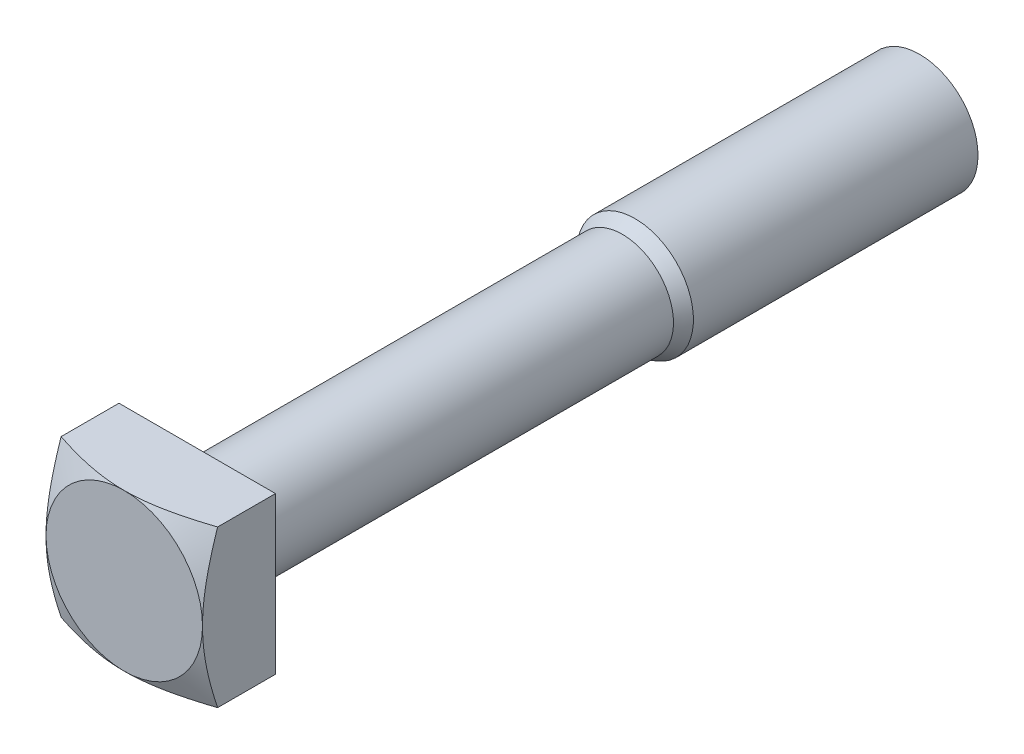
SolidWorks part; units mm, degrees
extrude "Base-Extrude" add sketch "Sketch1" along normal blind 15
sketch "Sketch1" plane through (0, 0, 0) normal (0, 0, 1) x (1, 0, 0)
  line L0 (-16.0867, 16.0867) -> (16.0867, -16.0867) construction
  line L1 (-16.0867, 16.0867) -> (16.0867, 16.0867)
  line L2 (-16.0867, 16.0867) -> (-16.0867, -16.0867)
  line L3 (-16.0867, -16.0867) -> (16.0867, -16.0867)
  line L4 (16.0867, 16.0867) -> (16.0867, -16.0867)
revolve "Boss-Revolve1" add sketch "Sketch2" angle 360 about L6
sketch "Sketch2" plane through (0, 0, 0) normal (0, 1, 0) x (1, 0, 0)
  line L0 (0, 0) -> (10.5, 0)
  line L1 (16.0867, 0) -> (-16.0867, 0) construction
  line L2 (10.5, 0) -> (10.5, 87.4019)
  line L3 (10.5, 87.4019) -> (12, 90)
  line L4 (12, 90) -> (12, 150)
  line L5 (12, 150) -> (0, 150)
  line L6 (0, 150) -> (0, 0) construction
  line L7 (0, 0) -> (0, 150)
cosmetic thread "Thread1" parameters "D1"=61.299, "D2"=21.402
ref_plane "front" through (0, 0, 0) normal (0, 0, 1) x (1, 0, 0)
ref_plane "top" through (0, 0, 0) normal (0, 1, 0) x (1, 0, 0)
ref_plane "right" through (0, 0, 0) normal (1, 0, 0) x (0, 0, -1)
sketch "dimension sketch" plane through (0, 0, 0) normal (0, 1, 0) x (1, 0, 0)
  line L0 (-22.75, 0) -> (22.75, 0)
  line L1 (22.75, 0) -> (22.75, 15)
  line L2 (22.75, 15) -> (10.9134, 15)
  line L3 (10.1134, 15.8) -> (10.1134, 97.5)
  line L4 (10.1134, 97.5) -> (12, 105)
  line L5 (12, 105) -> (12, 165)
  line L6 (12, 165) -> (-12, 165)
  line L7 (0, 0) -> (0, 165) construction
  line L8 (-22.75, 15) -> (-10.9134, 15)
  line L9 (-22.75, 0) -> (-22.75, 15)
  line L10 (-12, 105) -> (-12, 165)
  line L11 (-10.1134, 97.5) -> (-12, 105)
  line L12 (-10.1134, 15.8) -> (-10.1134, 97.5)
  arc A0 (10.9134, 15) -> (10.1134, 15.8) centre (10.9134, 15.8) cw
  arc A1 (-10.9134, 15) -> (-10.1134, 15.8) centre (-10.9134, 15.8) ccw
  point P9 (4.1274, 36)
  point P10 (12, 168)
sketch "Sketch4" plane through (0, 0, 15) normal (0, 0, 1) x (1, 0, 0)
  line L0 (16.0867, 16.0867) -> (-16.0867, 16.0867) construction
  circle A0 centre (0, 0) radius 16.0867
extrude "Cut-Extrude1" cut sketch "Sketch4" against normal through all draft 65 flip side to cut
fillet "Fillet1" radius 0.8 1 edges at (10.5, 0, 0)
sketch "Sketch3" plane through (0, 0, 0) normal (0, 1, 0) x (1, 0, 0)
  line L0 (9.402, 150) -> (12, 151.5)
  line L1 (12, 150) -> (-12, 150) construction
  line L2 (12, 151.5) -> (12, 148.5)
  line L3 (12, 148.5) -> (9.402, 150)
  line L4 (0, 0) -> (0, 4.1158) construction
  line L5 (0, 150) -> (0, 0) construction
  line L6 (12, 90) -> (12, 150) construction
revolve "Cut-Revolve1" cut sketch "Sketch3" angle 360 about L4
pattern_linear "LPattern1" [suppressed] count 21 spacing 3
equation "\"D1@Sketch1\" = \"e@dimension sketch\""
equation "\"D1@Base-Extrude\" = \"K@dimension sketch\""
equation "\"D1@Fillet1\" = \"r@dimension sketch\""
equation "\"D1@Sketch2\" = \"x@dimension sketch\""
equation "\"D2@Sketch2\"= \"L@dimension sketch\" "
equation "\"D4@Sketch2\"=\"B@dimension sketch\" "
equation "\"D3@Sketch2\" = \"D@dimension sketch\"/2"
equation "\"D3@LPattern1\" = \"P@dimension sketch\""
equation "\"D5@Sketch2\" = \"D3@Sketch2\" * 2 -3"
equation "\"D1@LPattern1\" = \"D4@Sketch2\" / \"D3@LPattern1\"+1"
equation "\"D3@Sketch3\" = \"D3@LPattern1\"*0.866"
equation "\"D1@Thread1\" = \"D4@Sketch2\" + \"D1@Sketch2\" / 2"
equation "\"D2@Thread1\" = \"D3@Sketch2\" * 2 - \"D3@Sketch3\""
